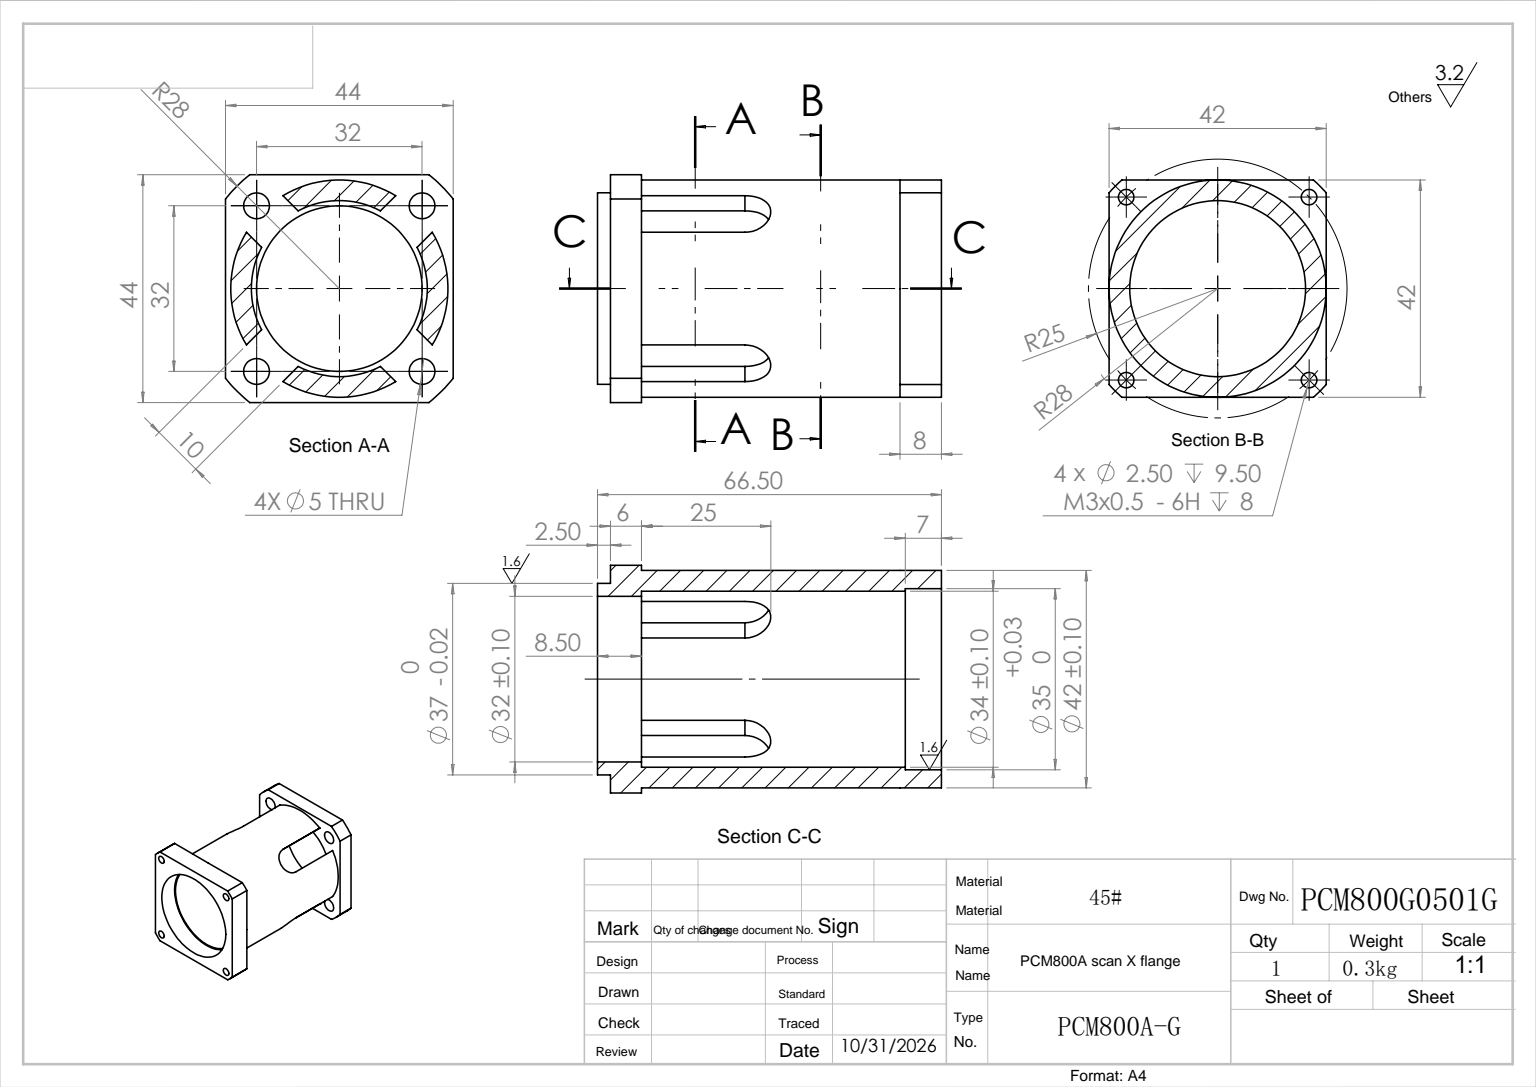
from build123d import *

# Parameters (mm, degrees)
SKETCH_1_R           = 21
SKETCH_1_R_2         = 17
EXTRUDE_1_DEPTH      = 50
SKETCH_3_W           = 44
SKETCH_3_H           = 44
EXTRUDE_2_DEPTH      = 6
SKETCH_4_R           = 2.5
CUT_EXTRUDE_2_DEPTH  = 6
SKETCH_5_W           = 42
SKETCH_5_H           = 42
EXTRUDE_3_DEPTH      = 8
SKETCH_6_R           = 18.5
EXTRUDE_4_DEPTH      = 2.5
CUT_EXTRUDE_3_REACH  = 75.418
SKETCH_7_R           = 17
SKETCH_8_R           = 17.5
CUT_EXTRUDE_4_DEPTH  = 7
M3X0_5_1_D           = 2.5
M3X0_5_1_DEPTH       = 9.5
M3X0_5_1_CBORE_D     = 3
M3X0_5_1_CBORE_DEPTH = 8
M3X0_5_1_TIP         = 0.751075774
CUT_EXTRUDE_6_DEPTH  = 91.112429775
CUT_EXTRUDE_7_DEPTH  = 91.112429775
CUT_EXTRUDE_8_REACH  = 75.418
SKETCH_13_R          = 16
SKETCH_14_OUTSIDE_W  = 64.214
SKETCH_14_OUTSIDE_H  = 64.214
SKETCH_14_OUTSIDE_R  = 28
CUT_EXTRUDE_9_DEPTH  = 74.418321964


with BuildPart() as part:
    # 草图1 → 拉伸1 (new body)
    with BuildSketch(Plane.XY):
        Circle(SKETCH_1_R)
        Circle(SKETCH_1_R_2, mode=Mode.SUBTRACT)
    extrude(amount=EXTRUDE_1_DEPTH)

    # 草图3 → 拉伸2 (add)
    with BuildSketch(Plane(origin=(0, 0, 0), x_dir=(-1, 0, 0), z_dir=(0, 0, -1))):
        Rectangle(SKETCH_3_W, SKETCH_3_H)
    extrude(amount=EXTRUDE_2_DEPTH)

    # 草图4 → 切除-拉伸2 (cut)
    with BuildSketch(Plane(origin=(0, 0, -6), x_dir=(-1, 0, 0), z_dir=(0, 0, -1))):
        with Locations((-16, 16)):
            Circle(SKETCH_4_R)
        with Locations(Location((16, 16, 0), (0, 0, 271.937166839))):
            Circle(SKETCH_4_R)
        with Locations((16, -16)):
            Circle(SKETCH_4_R)
        with Locations(Location((-16, -16, 0), (0, 0, 358.062833161))):
            Circle(SKETCH_4_R)
    extrude(amount=-CUT_EXTRUDE_2_DEPTH, mode=Mode.SUBTRACT)

    # 草图5 → 拉伸3 (add)
    with BuildSketch(Plane.XY.offset(50)):
        Rectangle(SKETCH_5_W, SKETCH_5_H)
    extrude(amount=EXTRUDE_3_DEPTH)

    # 草图6 → 拉伸4 (add)
    with BuildSketch(Plane(origin=(0, 0, -6), x_dir=(-1, 0, 0), z_dir=(0, 0, -1))):
        Circle(SKETCH_6_R)
    extrude(amount=EXTRUDE_4_DEPTH)

    # 草图7 → 切除-拉伸3 (cut, up to next)
    with BuildSketch(Plane.XY.offset(58), mode=Mode.PRIVATE) as cut_extrude_3_sk1:
        Circle(SKETCH_7_R)
    cut_extrude_3_tool1 = extrude(cut_extrude_3_sk1.sketch, amount=-CUT_EXTRUDE_3_REACH, mode=Mode.PRIVATE) & part.part
    add(cut_extrude_3_tool1.solids().sort_by_distance((0, 0, 58))[0], mode=Mode.SUBTRACT)

    # 草图8 → 切除-拉伸4 (cut)
    with BuildSketch(Plane.XY.offset(58)):
        Circle(SKETCH_8_R)
    extrude(amount=-CUT_EXTRUDE_4_DEPTH, mode=Mode.SUBTRACT)

    # M3x0.5 螺纹孔1
    with Locations(Plane(origin=(-17.67766953, 17.67766953, 58), x_dir=(1, 0, 0), z_dir=(0, 0, 1))):
        with Locations((0, 0), (35.35533906, 0), (0, -35.35533906), (35.35533906, -35.35533906)):
            CounterBoreHole(M3X0_5_1_D / 2, M3X0_5_1_CBORE_D / 2, M3X0_5_1_CBORE_DEPTH, depth=M3X0_5_1_DEPTH)
            with Locations((0, 0, -(M3X0_5_1_DEPTH + M3X0_5_1_TIP / 2))):  # 118° drill point
                Cone(0, M3X0_5_1_D / 2, M3X0_5_1_TIP, mode=Mode.SUBTRACT)

    # 草图11 → 切除-拉伸6 (cut, through all)
    with BuildSketch(Plane(origin=(21, 21, 58), x_dir=(0.7071067811865475, -0.7071067811865477, 0), z_dir=(-0.7071067811865477, -0.7071067811865475, 0))):
        with BuildLine():
            Line((-5, -38), (-5, -58))
            Line((-5, -58), (5, -58))
            Line((5, -58), (5, -38))
            ThreePointArc((5, -38), (0, -33), (-5, -38))
        make_face()
    extrude(amount=CUT_EXTRUDE_6_DEPTH, mode=Mode.SUBTRACT)

    # 草图12 → 切除-拉伸7 (cut, through all)
    with BuildSketch(Plane(origin=(21, -21, 58), x_dir=(0.7071067811865475, 0.7071067811865477, 0), z_dir=(0.7071067811865477, -0.7071067811865475, 0))):
        with BuildLine():
            Line((-5, -38), (-5, -58))
            Line((-5, -58), (5, -58))
            Line((5, -58), (5, -38))
            ThreePointArc((5, -38), (0, -33), (-5, -38))
        make_face()
    extrude(amount=-CUT_EXTRUDE_7_DEPTH, mode=Mode.SUBTRACT)

    # 草图13 → 切除-拉伸8 (cut, up to next)
    with BuildSketch(Plane(origin=(0, 0, -8.5), x_dir=(-1, 0, 0), z_dir=(0, 0, -1)), mode=Mode.PRIVATE) as cut_extrude_8_sk1:
        Circle(SKETCH_13_R)
    cut_extrude_8_tool1 = extrude(cut_extrude_8_sk1.sketch, amount=-CUT_EXTRUDE_8_REACH, mode=Mode.PRIVATE) & part.part
    add(cut_extrude_8_tool1.solids().sort_by_distance((0, 0, -8.5))[0], mode=Mode.SUBTRACT)

    # 草图14 outside → 切除-拉伸9 (cut, through all)
    with BuildSketch(Plane.XY.offset(58)):
        Rectangle(SKETCH_14_OUTSIDE_W, SKETCH_14_OUTSIDE_H)
        Circle(SKETCH_14_OUTSIDE_R, mode=Mode.SUBTRACT)
    extrude(amount=-CUT_EXTRUDE_9_DEPTH, mode=Mode.SUBTRACT)


solid = part.part
